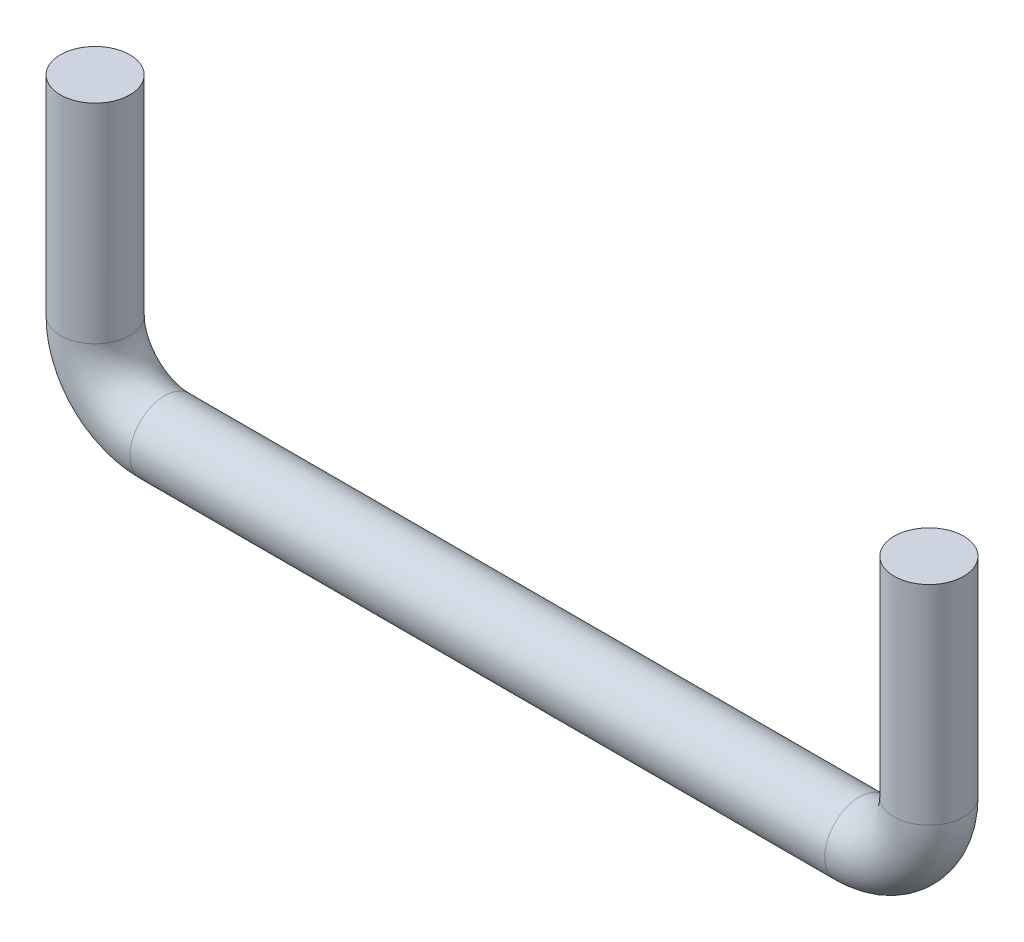
from build123d import *

# Parameters (mm, degrees)
SWEEP1_PROFILE_R = 5


with BuildPart() as part:
    # Sweep1: sweep along a path in Sketch1
    with BuildLine(Plane.XY) as sweep1_path:
        Line((-60, 40), (-60, 10))
        ThreePointArc((-60, 10), (-57.071067812, 2.928932188), (-50, 0))
        Line((-50, 0), (50, 0))
        ThreePointArc((50, 0), (57.071067812, 2.928932188), (60, 10))
        Line((60, 10), (60, 40))
    # Sweep1 profile (on start of the path) → Sweep1 (sweep)
    with BuildSketch(Plane(origin=(-60, 40, 0), x_dir=(-1, 0, 0), z_dir=(0, -1, 0))):
        Circle(SWEEP1_PROFILE_R)
    sweep(path=sweep1_path.line)


solid = part.part
